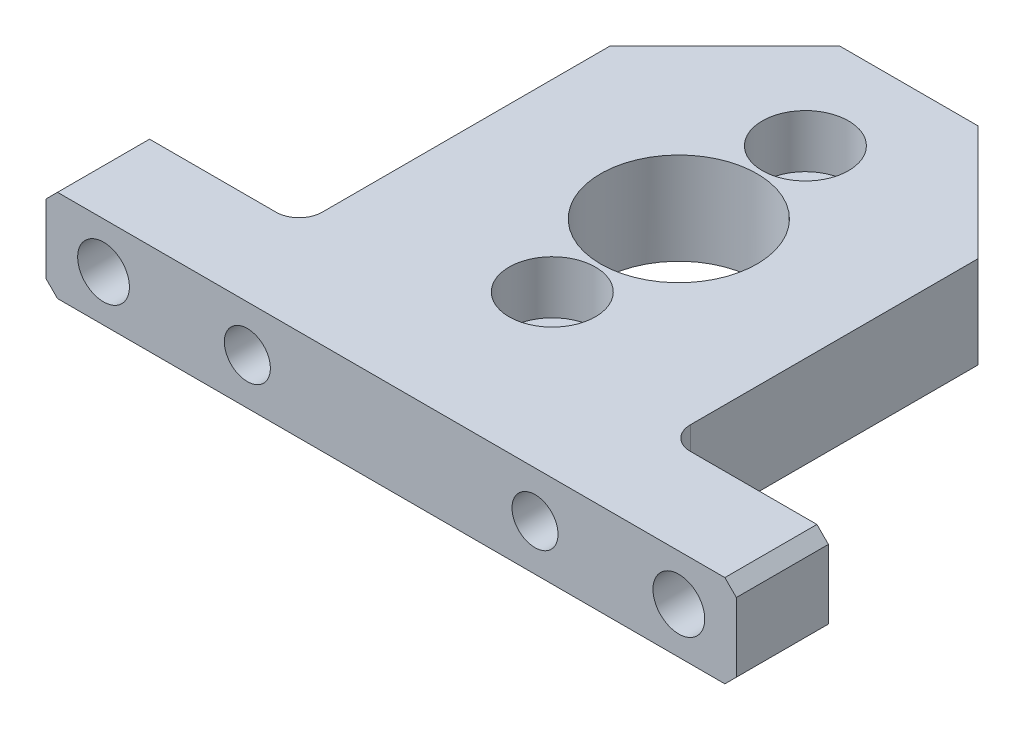
from build123d import *

# Parameters (mm, degrees)
EXTRUDE_1_DEPTH              = 4
CHAMFER_1_SIZE               = 1
CHAMFER_2_SIZE               = 10
CUT_EXTRUDE_1_REACH          = 56.672
SKETCH_2_R                   = 6.8
HOLE_WIZARD_M4_2_D           = 4.5
HOLE_WIZARD_M4_2_CBORE_D     = 7.5
HOLE_WIZARD_M4_2_CBORE_DEPTH = 4.6
F_4_0MM_1_D                  = 4
F_4_0MM_1_DEPTH              = 10
F_4_0MM_1_TIP                = 1.201721238
HOLE_WIZARD_M4_1_D           = 4.5


with BuildPart() as part:
    # 草图1 → 凸台-拉伸1 (new, symmetric)
    with BuildSketch(Plane(origin=(0, 0, 0), x_dir=(1, 0, 0), z_dir=(0, 1, 0))):
        with BuildLine():
            Line((-30, 0), (30, 0))
            Line((30, 0), (30, 8))
            Line((30, 8), (18, 8))
            ThreePointArc((18, 8), (16.585786438, 8.585786438), (16, 10))
            Line((16, 10), (16, 45))
            Line((16, 45), (-16, 45))
            Line((-16, 45), (-16, 10))
            ThreePointArc((-16, 10), (-16.585786438, 8.585786438), (-18, 8))
            Line((-18, 8), (-30, 8))
            Line((-30, 8), (-30, 0))
        make_face()
    extrude(amount=EXTRUDE_1_DEPTH, both=True)

    # 倒角1
    chamfer_1_edges = [part.edges().sort_by_distance(p)[0] for p in [
        (30, 4, -4),
        (30, -4, -4),
        (-30, -4, -4),
        (-30, 4, -4),
    ]]
    chamfer(chamfer_1_edges, length=CHAMFER_1_SIZE)

    # 倒角2
    chamfer_2_edges = [part.edges().sort_by_distance(p)[0] for p in [
        (-16, 0, -45),
        (16, 0, -45),
    ]]
    chamfer(chamfer_2_edges, length=CHAMFER_2_SIZE)

    # 草图2 → 切除-拉伸1 (cut, up to next)
    with BuildSketch(Plane(origin=(0, 4, 0), x_dir=(1, 0, 0), z_dir=(0, 1, 0)), mode=Mode.PRIVATE) as cut_extrude_1_sk1:
        with Locations(Location((0, 25, 0), (0, 0, 270))):
            Circle(SKETCH_2_R)
    cut_extrude_1_tool1 = extrude(cut_extrude_1_sk1.sketch, amount=-CUT_EXTRUDE_1_REACH, mode=Mode.PRIVATE) & part.part
    add(cut_extrude_1_tool1.solids().sort_by_distance((0, 4, -25))[0], mode=Mode.SUBTRACT)

    # M4 六角圆柱头螺钉的柱形沉头孔2 (through all)
    with Locations(Plane(origin=(0, 4, 0), x_dir=(1, 0, 0), z_dir=(0, 1, 0))):
        with Locations((0, 36), (0, 14)):
            CounterBoreHole(HOLE_WIZARD_M4_2_D / 2, HOLE_WIZARD_M4_2_CBORE_D / 2, HOLE_WIZARD_M4_2_CBORE_DEPTH)

    # Ø4.0mm 暗销孔1
    with Locations(Plane.XY):
        with Locations((-12.5, 0), (12.5, 0)):
            Hole(F_4_0MM_1_D / 2, depth=F_4_0MM_1_DEPTH)
            with Locations((0, 0, -(F_4_0MM_1_DEPTH + F_4_0MM_1_TIP / 2))):  # 118° drill point
                Cone(0, F_4_0MM_1_D / 2, F_4_0MM_1_TIP, mode=Mode.SUBTRACT)

    # M4 间隙孔1 (through all)
    with Locations(Plane(origin=(0, 0, -8), x_dir=(-1, 0, 0), z_dir=(0, 0, -1))):
        with Locations((-25, 0), (25, 0)):
            Hole(HOLE_WIZARD_M4_1_D / 2)


solid = part.part
